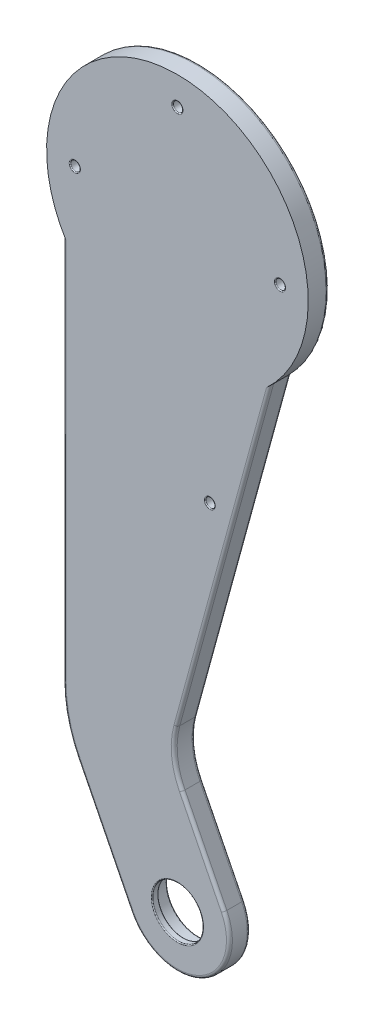
SolidWorks part; units mm, degrees
ref_plane "Front Plane" through (0, 0, 0) normal (0, 0, 1) x (1, 0, 0)
ref_plane "Top Plane" through (0, 0, 0) normal (0, 1, 0) x (1, 0, 0)
ref_plane "Right Plane" through (0, 0, 0) normal (1, 0, 0) x (0, 0, -1)
sketch "Sketch1" plane through (0, 0, 0) normal (0, 0, 1) x (1, 0, 0)
  line L2 (0, 0) -> (34.5, 0) construction
  line L3 (0, -191.5) -> (0, -200) construction
  line L4 (-38.4041, -21.4739) -> (-38.4041, -162.4687)
  line L5 (-38.4041, -162.4687) -> (-15.6424, -207.8463)
  line L6 (-30.7621, -72.1726) -> (-20.8155, -71.1406) construction
  line L7 (31.3784, -30.8447) -> (-2.7253, -155.5358)
  line L8 (-2.7253, -155.5358) -> (15.6424, -192.1537)
  circle A10 centre (0, -200) radius 8.5
  arc A11 (-15.6424, -207.8463) -> (15.6424, -192.1537) centre (0, -200) ccw
  circle A31 centre (-34.5, 0) radius 1.6
  circle A33 centre (0, 34.5) radius 1.6
  circle A35 centre (34.5, 0) radius 1.6
  arc A37 (31.3784, -30.8447) -> (-38.4041, -21.4739) centre (0, 0) ccw
  point P28 (0, -100)
  point P33 (0, 0)
  dimension "D1" = 88
  dimension "D2" = 200
  dimension "D5" = 17
  dimension "D6" = 35
  dimension "D4" = 10
extrude "Boss-Extrude1" add sketch "Sketch1" along normal blind 7
fillet "Fillet1" radius 25 1 edges at (-2.7253, -155.5358, 3.5)
fillet "Fillet2" radius 45 1 edges at (-38.4041, -162.4687, 3.5)
sketch "Sketch2" plane through (0, 0, 0) normal (0, 0, -1) x (-1, 0, 0)
  circle A0 centre (0, -200) radius 10.5
  dimension "D1" = 21
extrude "Cut-Extrude1" cut sketch "Sketch2" against normal blind 5
sketch "Sketch3" plane through (0, 0, 7) normal (0, 0, 1) x (1, 0, 0)
  line L0 (31.3784, -30.8447) -> (-0.1979, -146.2948) construction
  circle A0 centre (10.9092, -75.3606) radius 1.55
  arc A1 (-0.1979, -146.2948) -> (1.5701, -164.0992) centre (23.9165, -152.8902) ccw construction
  point P7 (-0.9612, -155.3606)
  dimension "D1" = 3.1
  dimension "D2" = 8
  dimension "D3" = 80
extrude "Cut-Extrude2" cut sketch "Sketch3" against normal up to next
sketch "Sketch5" plane through (0, 0, 0) normal (0, 0, -1) x (-1, 0, 0)
  circle A0 centre (0, 34.5) radius 3.5
  circle A1 centre (-10.9092, -75.3606) radius 3.5
  circle A2 centre (34.5, 0) radius 3.5
  circle A4 centre (-34.5, 0) radius 3.5
  circle A5 centre (0, -34.5) radius 3.5 [skipped]
  dimension "D1" = 7
  dimension "D2" = 7
  dimension "D3" = 4
extrude "Cut-Extrude4" cut sketch "Sketch5" against normal blind 1.8
fillet "Fillet3" radius 1 15 edges at (7.8463, -215.6424, 7) (8.6063, -178.1264, 7) (-24.6349, -189.9189, 7) (-0.9612, -155.3606, 7) (-37.1936, -162.1822, 7) (15.5903, -88.5698, 7) (-38.4041, -86.6445, 7) (15.5903, -88.5698, 0) (-0.9612, -155.3606, 0) (8.6063, -178.1264, 0) (7.8463, -215.6424, 0) (-24.6349, -189.9189, 0) (-37.1936, -162.1822, 0) (5.8561, 43.6086, 0) (-38.4041, -86.6445, 0)
fillet "Fillet5" radius 0.3 10 edges at (12.4592, -75.3606, 7) (36.1, 0, 7) (-32.9, 0, 7) (1.6, 34.5, 7) (8.5, -200, 7) (-10.5, -200, 0) (7.4092, -75.3606, 0) (-38, 0, 0) (31, 0, 0) (-3.5, 34.5, 0)
fillet "Fillet6" radius 0.1 10 edges at (-10.5, -200, 5) (-8.5, -200, 5) (9.3592, -75.3606, 1.8) (7.4092, -75.3606, 1.8) (-36.1, 0, 1.8) (-38, 0, 1.8) (32.9, 0, 1.8) (31, 0, 1.8) (-1.6, 34.5, 1.8) (-3.5, 34.5, 1.8)
